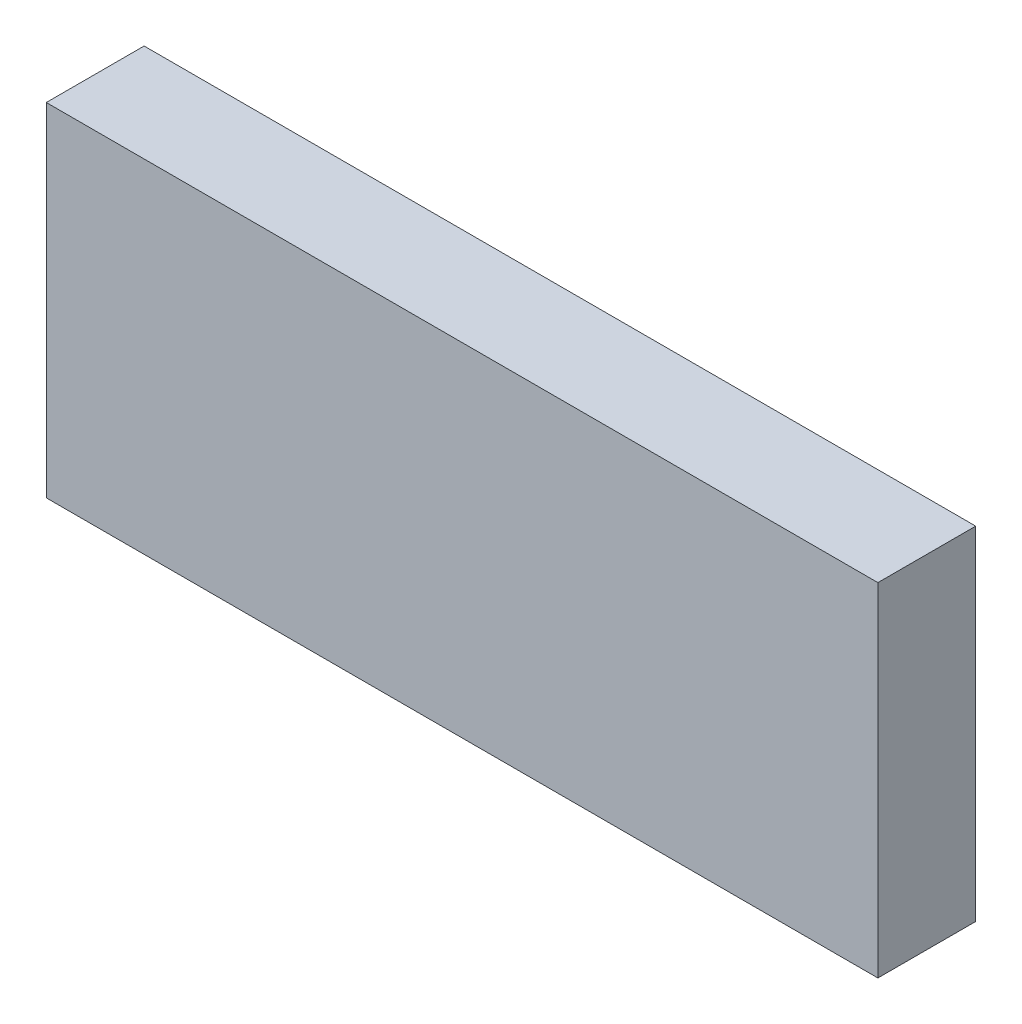
SolidWorks part; units mm, degrees
material "1023 碳钢板 (SS)"
ref_plane "前视基准面" through (0, 0, 0) normal (0, 0, 1) x (1, 0, 0)
ref_plane "上视基准面" through (0, 0, 0) normal (0, 1, 0) x (1, 0, 0)
ref_plane "右视基准面" through (0, 0, 0) normal (1, 0, 0) x (0, 0, -1)
sketch "草图1" plane through (0, 0, 0) normal (0, 0, 1) x (1, 0, 0)
  line L1 (85, 35) -> (-85, 35)
  line L2 (85, 35) -> (85, -35)
  line L3 (85, -35) -> (-85, -35)
  line L4 (-85, 35) -> (-85, -35)
  line L5 (85, 35) -> (-85, -35) construction
  line L6 (85, -35) -> (-85, 35) construction
  point P0 (0, 0)
  dimension "D1" = 170
  dimension "D2" = 70
extrude "凸台-拉伸1" add sketch "草图1" along normal blind 20
